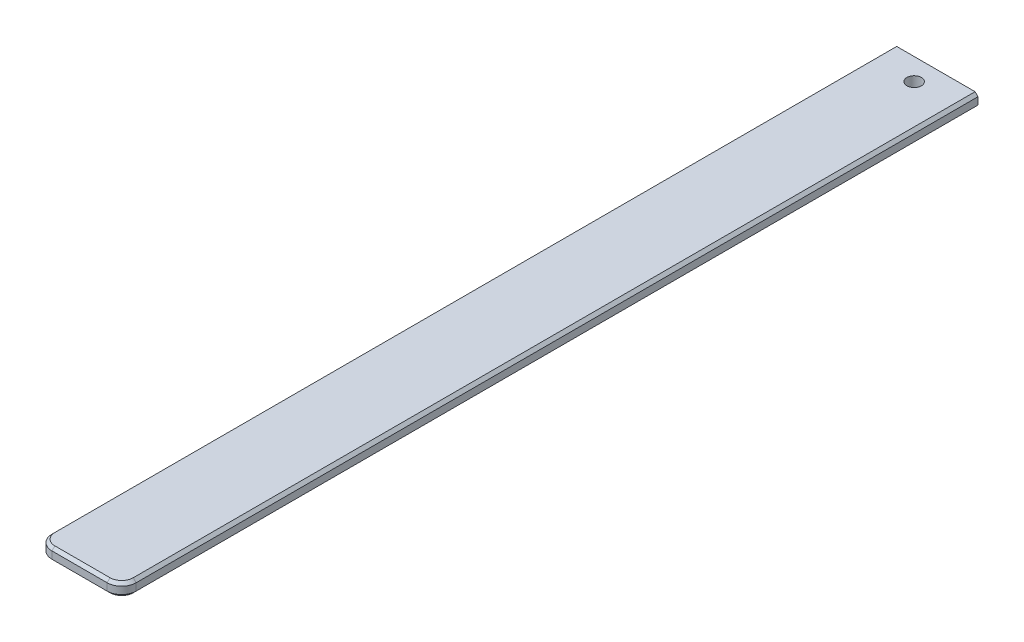
SolidWorks part; units mm, degrees
material "S136"
ref_plane "Front Plane" through (0, 0, 0) normal (0, 0, 1) x (1, 0, 0)
ref_plane "Top Plane" through (0, 0, 0) normal (0, 1, 0) x (1, 0, 0)
ref_plane "Right Plane" through (0, 0, 0) normal (1, 0, 0) x (0, 0, -1)
sketch "Sketch1" plane through (0, 0, 0) normal (0, 1, 0) x (1, 0, 0)
  line L1 (-2.25, -1.5) -> (2.25, -1.5)
  line L2 (-2.25, -1.5) -> (-2.25, 1.5)
  line L3 (-2.25, 1.5) -> (2.25, 1.5)
  line L4 (2.25, -1.5) -> (2.25, 1.5)
  line L5 (-2.25, -1.5) -> (2.25, 1.5) construction
  line L6 (-2.25, 1.5) -> (2.25, -1.5) construction
  point P0 (0, 0)
  dimension "D1" = 4.5
  dimension "D2" = 3
extrude "Boss-Extrude1" add sketch "Sketch1" along normal blind 8
sketch "Sketch2" plane through (0, 0, 1.5) normal (0, 0, 1) x (1, 0, 0)
  line L0 (0, 8) -> (0, 0) construction
  line L1 (-2.25, 8) -> (2.25, 8) construction
  line L2 (-2.25, 0) -> (2.25, 0) construction
  line L3 (-1.45, 0.65) -> (1.45, 0.65)
  line L4 (-1.45, 0.65) -> (-1.45, 0.2)
  line L5 (-1.45, 0.2) -> (1.45, 0.2)
  line L6 (1.45, 0.65) -> (1.45, 0.2)
  line L7 (-1.45, 0.65) -> (1.45, 0.2) construction
  line L8 (-1.45, 0.2) -> (1.45, 0.65) construction
  point P5 (0, 0.425)
  dimension "D1" = 2.9
  dimension "D2" = 0.45
  dimension "D3" = 0.2
extrude "Boss-Extrude2" add sketch "Sketch2" along normal blind 26.5
fillet "Fillet1" radius 0.5 2 edges at (-1.45, 0.425, 28) (1.45, 0.425, 28)
chamfer "Chamfer1" distance 1 distance2 1 1 edges at (0, 8, 1.5)
chamfer "Chamfer2" distance 0.1 angle 45 10 edges at (1.45, 0.65, 14.5) (1.3036, 0.65, 27.8536) (0, 0.65, 28) (-1.3036, 0.65, 27.8536) (-1.45, 0.65, 14.5) (1.45, 0.2, 14.5) (1.3036, 0.2, 27.8536) (0, 0.2, 28) (-1.3036, 0.2, 27.8536) (-1.45, 0.2, 14.5)
sketch "Sketch3" plane through (0, 0, 1.5) normal (0, 0, 1) x (1, 0, 0)
  line L0 (0, 7) -> (0, 0.65) construction
  line L1 (2.25, 7) -> (-2.25, 7) construction
  line L2 (-0.95, 0.65) -> (0.95, 0.65) construction
  circle A0 centre (0, 3.825) radius 1.525
  dimension "D1" = 3.05
extrude "Cut-Extrude1" cut sketch "Sketch3" against normal blind 2.1
sketch "Sketch5" plane through (0, 0, -0.6) normal (0, 0, 1) x (1, 0, 0)
  circle A0 centre (0, 3.825) radius 0.6
  dimension "D1" = 1.2
extrude "Cut-Extrude2" cut sketch "Sketch5" against normal blind 2.1
sketch "Sketch6" plane through (2.25, 0, 0) normal (1, 0, 0) x (0, 0, -1)
  line L5 (1.5, 8) -> (-0.5, 8)
  line L6 (-0.5, 8) -> (-1.5, 7)
  line L7 (-1.5, 7) -> (-1.5, 0)
  line L8 (-1.5, 0) -> (1.5, 0)
  line L9 (1.5, 0) -> (1.5, 8)
  line L10 (1.5, 8) -> (-0.5, 8)
  line L11 (-0.5, 8) -> (-1.5, 7)
  line L12 (-1.5, 7) -> (-1.5, 0)
  line L13 (-1.5, 0) -> (1.5, 0)
  line L14 (1.5, 0) -> (1.5, 8)
  dimension "D1" = 0
extrude "Cut-Extrude3" cut sketch "Sketch6" against normal through all
sketch "Sketch7" plane through (0, 0, 1.5) normal (0, 0, -1) x (-1, 0, 0)
  line L8 (1.45, 0.55) -> (1.35, 0.65)
  line L9 (1.35, 0.65) -> (-1.35, 0.65)
  line L10 (-1.35, 0.65) -> (-1.45, 0.55)
  line L11 (-1.45, 0.55) -> (-1.45, 0.3)
  line L12 (-1.45, 0.3) -> (-1.35, 0.2)
  line L13 (-1.35, 0.2) -> (1.35, 0.2)
  line L14 (1.35, 0.2) -> (1.45, 0.3)
  line L15 (1.45, 0.3) -> (1.45, 0.55)
  line L16 (1.45, 0.55) -> (1.35, 0.65)
  line L17 (1.35, 0.65) -> (-1.35, 0.65)
  line L18 (-1.35, 0.65) -> (-1.45, 0.55)
  line L19 (-1.45, 0.55) -> (-1.45, 0.3)
  line L20 (-1.45, 0.3) -> (-1.35, 0.2)
  line L21 (-1.35, 0.2) -> (1.35, 0.2)
  line L22 (1.35, 0.2) -> (1.45, 0.3)
  line L23 (1.45, 0.3) -> (1.45, 0.55)
  dimension "D1" = 0
extrude "Boss-Extrude3" add sketch "Sketch7" along normal blind 3
sketch "Sketch8" plane through (0, 0.2, 0) normal (0, -1, 0) x (1, 0, 0)
  line L0 (1.35, -1.5) -> (-1.35, -1.5) construction
  line L1 (-1.45, -1.5) -> (-1.45, 27.5) construction
  circle A0 centre (0, -0.75) radius 0.25
  dimension "D1" = 0.5
  dimension "D2" = 0.75
  dimension "D3" = 1.45
extrude "Cut-Extrude4" cut sketch "Sketch8" against normal blind 3
equation "\"code1\"= \"图名分离代码\""
equation "\"code2\"= \"图号分离代码\""
